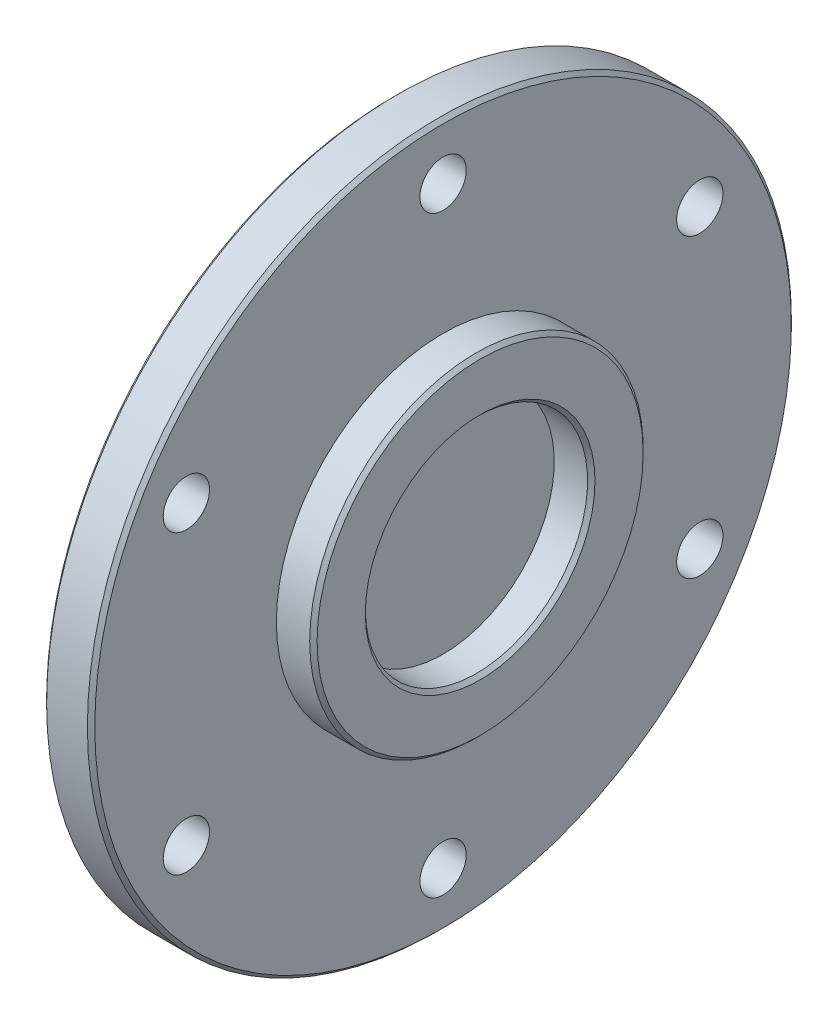
from build123d import *

# Parameters (mm, degrees)
SKETCH_2_R               = 6.25
CUT_EXTRUDE_1_DEPTH      = 137.304805491
PATTERN_CIRCULAR_1_COUNT = 6
CHAMFER_1_SIZE           = 1


with BuildPart() as part:
    # 草图1 → 旋转1 (revolve)
    with BuildSketch(Plane.XY, mode=Mode.PRIVATE) as revolve_1_sk:
        Polygon((0, 0), (0, 95), (13, 95), (13, 45), (23, 45), (23, 30), (13, 30), (13, 0), align=None)
    revolve(revolve_1_sk.sketch.rotate(Axis((0, 0, 0), (1, 0, 0)), 90), axis=Axis((0, 0, 0), (1, 0, 0)))

    # 草图2 → 切除-拉伸1 (cut, through all)
    with BuildSketch(Plane.ZY):
        with Locations((0, 80)):
            Circle(SKETCH_2_R)
    cut_extrude_1 = extrude(amount=-CUT_EXTRUDE_1_DEPTH, mode=Mode.SUBTRACT)

    # 阵列(圆周)1: 切除-拉伸1 ×6 about axis
    pattern_circular_1_axis = Axis((0, 0, 0), (1, 0, 0))
    for i in range(1, PATTERN_CIRCULAR_1_COUNT):
        add(cut_extrude_1.rotate(pattern_circular_1_axis, i * 360 / PATTERN_CIRCULAR_1_COUNT), mode=Mode.SUBTRACT)

    # 倒角1
    chamfer_1_edges = [part.edges().sort_by_distance(p)[0] for p in [
        (23, 0, -30),
        (23, 0, -45),
        (13, 0, -95),
        (0, 0, -95),
    ]]
    chamfer(chamfer_1_edges, length=CHAMFER_1_SIZE)


solid = part.part
